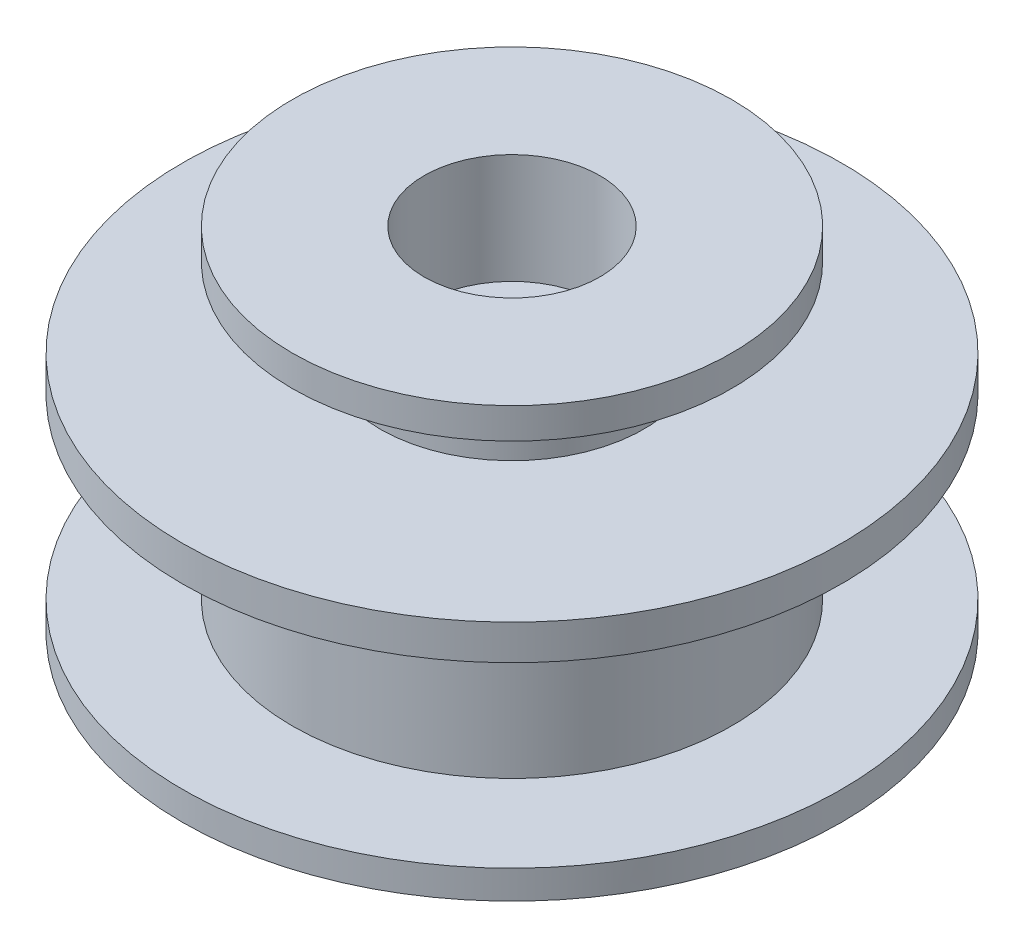
from build123d import *

# Parameters (mm, degrees)
SKETCH1_R           = 7.5
BOSS_EXTRUDE1_DEPTH = 4
SKETCH3_W           = 3
SKETCH3_H           = 3.25
SKETCH4_R           = 5
BOSS_EXTRUDE2_DEPTH = 8
SKETCH5_W           = 2
SKETCH5_H           = 1.8
SKETCH6_R           = 2
CUT_EXTRUDE1_DEPTH  = 14.285330256
CUT_EXTRUDE3_START  = -2
SKETCH7_R           = 8.572097994
SKETCH7_R_2         = 5
CUT_EXTRUDE3_DEPTH  = 2
BOSS_EXTRUDE3_START = -0.8
SKETCH8_R           = 7.5
BOSS_EXTRUDE3_DEPTH = 0.8


with BuildPart() as part:
    # Sketch1 → Boss-Extrude1 (new body)
    with BuildSketch(Plane(origin=(0, 0, 0), x_dir=(1, 0, 0), z_dir=(0, 1, 0))):
        with Locations(Location((0, 0, 0), (0, 0, 270))):
            Circle(SKETCH1_R)
    extrude(amount=BOSS_EXTRUDE1_DEPTH)

    # Sketch3 → Cut-Revolve1 (revolve, cut)
    with BuildSketch(Plane.XY, mode=Mode.PRIVATE) as cut_revolve1_sk:
        with Locations((6, 2.275)):
            Rectangle(SKETCH3_W, SKETCH3_H)
    revolve(cut_revolve1_sk.sketch.rotate(Axis((0, 0, 0), (0, 1, 0)), 90), axis=Axis((0, 0, 0), (0, 1, 0)), mode=Mode.SUBTRACT)

    # Sketch4 → Boss-Extrude2 (add)
    with BuildSketch(Plane(origin=(0, 0, 0), x_dir=(1, 0, 0), z_dir=(0, 1, 0))):
        with Locations(Location((0, 0, 0), (0, 0, 90))):
            Circle(SKETCH4_R)
    extrude(amount=BOSS_EXTRUDE2_DEPTH)

    # Sketch5 → Cut-Revolve2 (revolve, cut)
    with BuildSketch(Plane.XY, mode=Mode.PRIVATE) as cut_revolve2_sk:
        with Locations((4, 6.4)):
            Rectangle(SKETCH5_W, SKETCH5_H)
    revolve(cut_revolve2_sk.sketch.rotate(Axis((0, 4, 0), (0, 1, 0)), 90), axis=Axis((0, 4, 0), (0, 1, 0)), mode=Mode.SUBTRACT)

    # Sketch6 → Cut-Extrude1 (cut, through all)
    with BuildSketch(Plane(origin=(0, 8, 0), x_dir=(1, 0, 0), z_dir=(0, 1, 0))):
        with Locations(Location((0, 0, 0), (0, 0, 270))):
            Circle(SKETCH6_R)
    extrude(amount=-CUT_EXTRUDE1_DEPTH, mode=Mode.SUBTRACT)

    # Sketch7 → Cut-Extrude3 (cut)
    with BuildSketch(Plane(origin=(0, 4, 0), x_dir=(1, 0, 0), z_dir=(0, 1, 0)).offset(CUT_EXTRUDE3_START)):
        Circle(SKETCH7_R)
        with Locations(Location((0, 0, 0), (0, 0, 90))):
            Circle(SKETCH7_R_2, mode=Mode.SUBTRACT)
    extrude(amount=CUT_EXTRUDE3_DEPTH, mode=Mode.SUBTRACT)

    # Sketch8 → Boss-Extrude3 (add)
    with BuildSketch(Plane(origin=(0, 5.5, 0), x_dir=(1, 0, 0), z_dir=(0, 1, 0)).offset(BOSS_EXTRUDE3_START)):
        with Locations(Location((0, 0, 0), (0, 0, 270))):
            Circle(SKETCH8_R)
    extrude(amount=BOSS_EXTRUDE3_DEPTH)


solid = part.part
